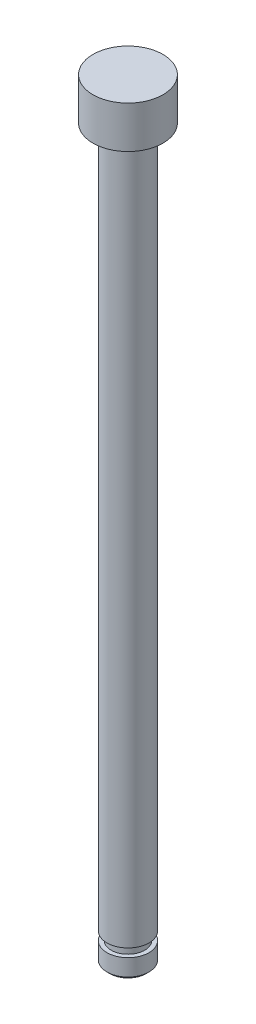
from build123d import *

# Parameters (mm, degrees)
SKETCH1_R           = 0.75
BOSS_EXTRUDE1_DEPTH = 26
SKETCH2_R           = 1.25
BOSS_EXTRUDE2_DEPTH = 1.5
SKETCH3_OUTSIDE_W   = 10.046
SKETCH3_OUTSIDE_H   = 10.046
SKETCH3_OUTSIDE_R   = 0.6
CUT_EXTRUDE1_DEPTH  = 0.3
CHAMFER1_SIZE       = 0.1


with BuildPart() as part:
    # Sketch1 → Boss-Extrude1 (new body)
    with BuildSketch(Plane(origin=(0, 0, 0), x_dir=(1, 0, 0), z_dir=(0, 1, 0))):
        with Locations(Location((0, 0, 0), (0, 0, 270))):
            Circle(SKETCH1_R)
    extrude(amount=BOSS_EXTRUDE1_DEPTH)

    # Sketch2 → Boss-Extrude2 (add)
    with BuildSketch(Plane(origin=(0, 26, 0), x_dir=(1, 0, 0), z_dir=(0, 1, 0))):
        with Locations(Location((0, 0, 0), (0, 0, 270))):
            Circle(SKETCH2_R)
    extrude(amount=BOSS_EXTRUDE2_DEPTH)

    # Sketch3 outside → Cut-Extrude1 (cut)
    with BuildSketch(Plane(origin=(0, 1, 0), x_dir=(-1, 0, 0), z_dir=(0, -1, 0))):
        Rectangle(SKETCH3_OUTSIDE_W, SKETCH3_OUTSIDE_H)
        with Locations(Location((0, 0, 0), (0, 0, 90))):
            Circle(SKETCH3_OUTSIDE_R, mode=Mode.SUBTRACT)
    extrude(amount=CUT_EXTRUDE1_DEPTH, mode=Mode.SUBTRACT)

    # Chamfer1
    chamfer1_edges = [part.edges().sort_by_distance(p)[0] for p in [
        (0, 0, -0.75),
    ]]
    chamfer(chamfer1_edges, length=CHAMFER1_SIZE)


solid = part.part
